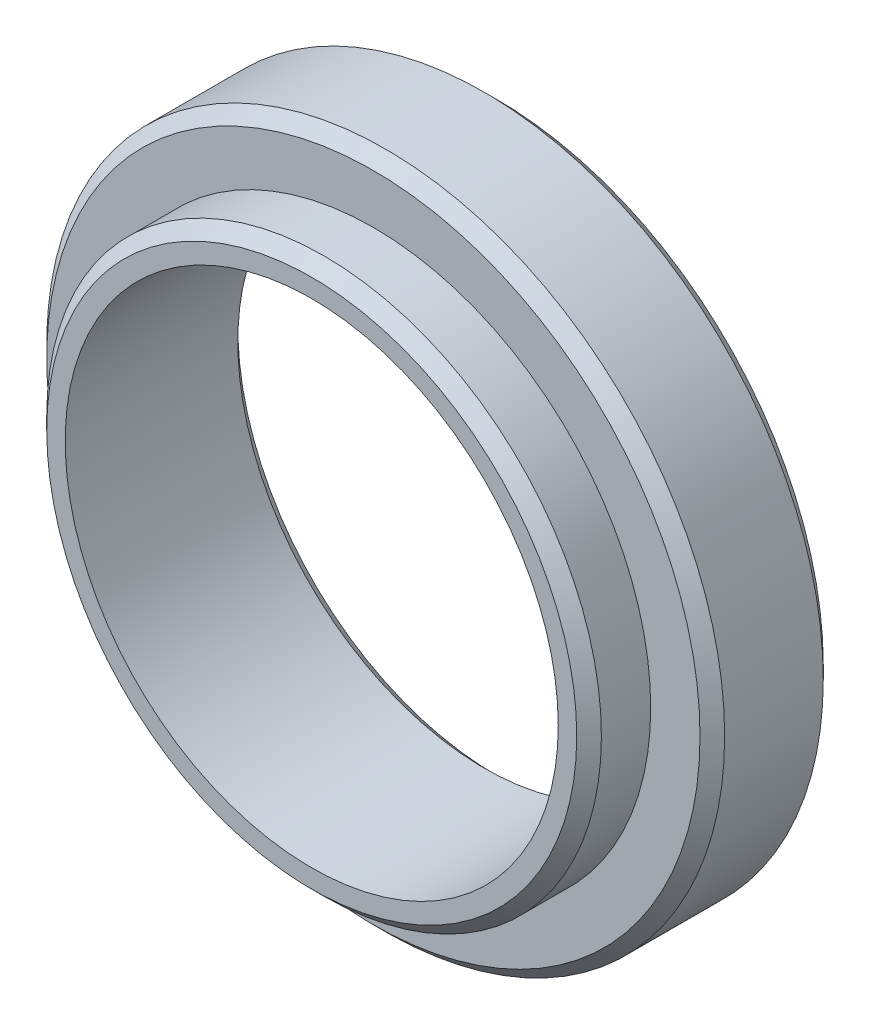
SolidWorks part; units mm, degrees
ref_plane "Front Plane" through (0, 0, 0) normal (0, 0, 1) x (1, 0, 0)
ref_plane "Top Plane" through (0, 0, 0) normal (0, 1, 0) x (1, 0, 0)
ref_plane "Right Plane" through (0, 0, 0) normal (1, 0, 0) x (0, 0, -1)
sketch "Sketch1" plane through (0, 0, 0) normal (0, 0, 1) x (1, 0, 0)
  circle A0 centre (0, 0) radius 27.5
  circle A1 centre (0, 0) radius 20
  dimension "D1" = 55
  dimension "D2" = 40
extrude "Boss-Extrude1" add sketch "Sketch1" along normal blind 15
sketch "Sketch2" plane through (0, 0, 15) normal (0, 0, 1) x (1, 0, 0)
  circle A0 centre (0, 0) radius 27.5
  circle A1 centre (0, 0) radius 22.5
  dimension "D1" = 45
extrude "Cut-Extrude1" cut sketch "Sketch2" against normal blind 5
chamfer "Chamfer1" distance 1 4 edges at (20, 0, 0) (27.5, 0, 0) (27.5, 0, 10) (22.5, 0, 15)
